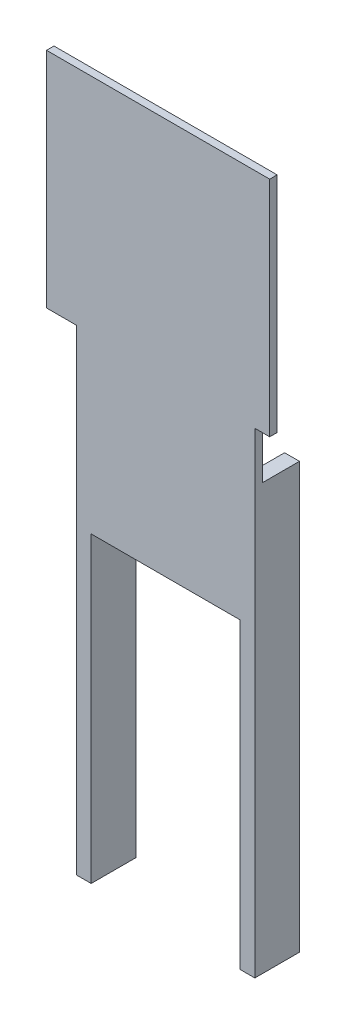
SolidWorks part; units mm, degrees
ref_plane "Front Plane" through (0, 0, 0) normal (0, 0, 1) x (1, 0, 0)
ref_plane "Top Plane" through (0, 0, 0) normal (0, 1, 0) x (1, 0, 0)
ref_plane "Right Plane" through (0, 0, 0) normal (1, 0, 0) x (0, 0, -1)
sketch "Sketch1" plane through (0, 0, 0) normal (0, 0, 1) x (1, 0, 0)
  line L2 (-60, 40) -> (-60, -80)
  line L3 (-60, -80) -> (60, -80)
  line L4 (60, 40) -> (60, -80)
  line L5 (-51.4286, 68.5714) -> (-30, 40) construction
  line L6 (-60, -80) -> (0, 0) construction
  line L7 (-80, 190) -> (70, 190)
  line L8 (-80, 190) -> (-80, 40)
  line L9 (-80, 40) -> (-60, 40)
  line L10 (70, 190) -> (70, 40)
  line L11 (-80, 190) -> (30, 80) construction
  line L12 (-60, 60) -> (-51.4286, 68.5714) construction
  line L13 (-40, 80) -> (70, 190) construction
  line L14 (60, 40) -> (70, 40)
  line L15 (0, 0) -> (60, -80) construction
  line L17 (60, 50) -> (70, 40) construction
  point P0 (0, 0)
  point P6 (-5, 115)
  dimension "D1" = 150
  dimension "D2" = 150
  dimension "D3" = 120
  dimension "D4" = 120
  dimension "D5" = 10
  dimension "D6" = 80
extrude "Boss-Extrude1" add sketch "Sketch1" along normal blind 5
sketch "Sketch2" plane through (0, 0, 5) normal (0, 0, 1) x (1, 0, 0)
  line L0 (60, -80) -> (60, 40) construction
  line L1 (60, 5.7578) -> (50, 5.7578)
  line L2 (60, 5.7578) -> (60, -280)
  line L3 (60, -280) -> (50, -280)
  line L4 (50, 5.7578) -> (50, -280)
  line L6 (-60, 40) -> (-60, -80) construction
  line L7 (-60, 33.599) -> (-50, 33.599)
  line L8 (-60, 33.599) -> (-60, -280)
  line L9 (-60, -280) -> (-50, -280)
  line L10 (-50, 33.599) -> (-50, -280)
  line L11 (-60, -80) -> (60, -80) construction
  dimension "D1" = 100
  dimension "D2" = 0
  dimension "D3" = 10
  dimension "D4" = 200
extrude "Boss-Extrude2" add sketch "Sketch2" against normal blind 30
chamfer "Chamfer1" distance 3.5 angle 45 1 edges at (0, -80, 5)
